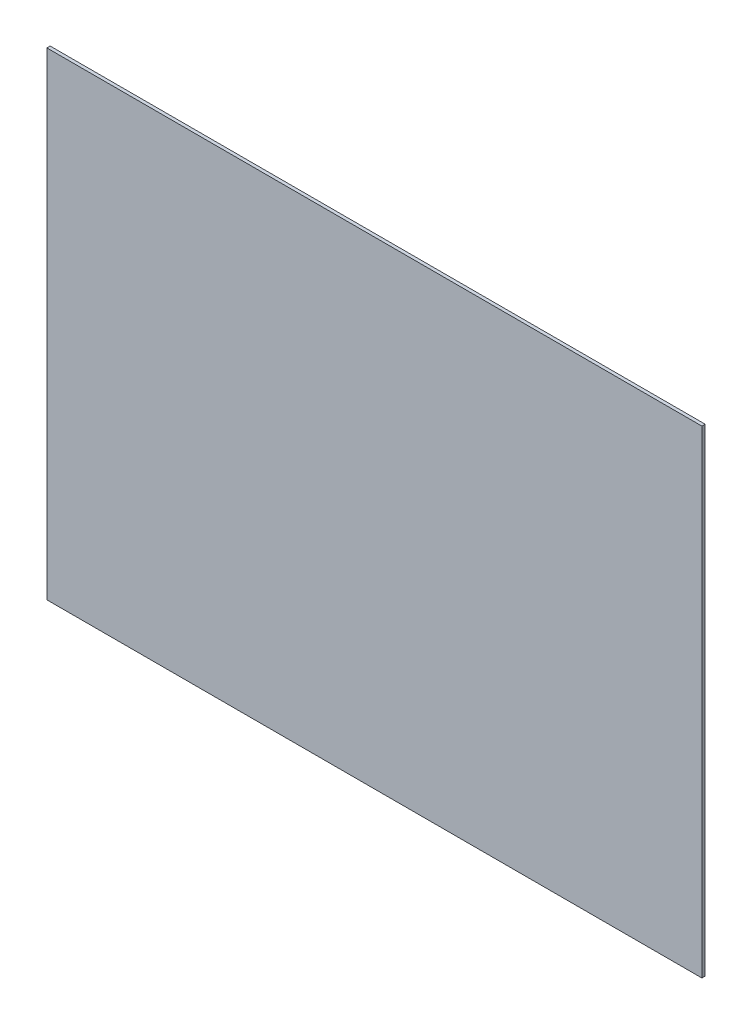
SolidWorks part; units mm, degrees
material "PMMA(有机玻璃)"
ref_plane "前视" through (0, 0, 0) normal (0, 0, 1) x (1, 0, 0)
ref_plane "上视" through (0, 0, 0) normal (0, 1, 0) x (1, 0, 0)
ref_plane "右视" through (0, 0, 0) normal (1, 0, 0) x (0, 0, -1)
sketch "草图1" plane through (0, 0, 0) normal (0, 0, 1) x (1, 0, 0)
  line L1 (-499.5, 364.5) -> (499.5, 364.5)
  line L2 (-499.5, 364.5) -> (-499.5, -364.5)
  line L3 (-499.5, -364.5) -> (499.5, -364.5)
  line L4 (499.5, 364.5) -> (499.5, -364.5)
  line L5 (-499.5, 364.5) -> (499.5, -364.5) construction
  line L6 (-499.5, -364.5) -> (499.5, 364.5) construction
  point P0 (0, 0)
  dimension "D1" = 729
  dimension "D2" = 999
extrude "凸台-拉伸1" add sketch "草图1" along normal blind 5
